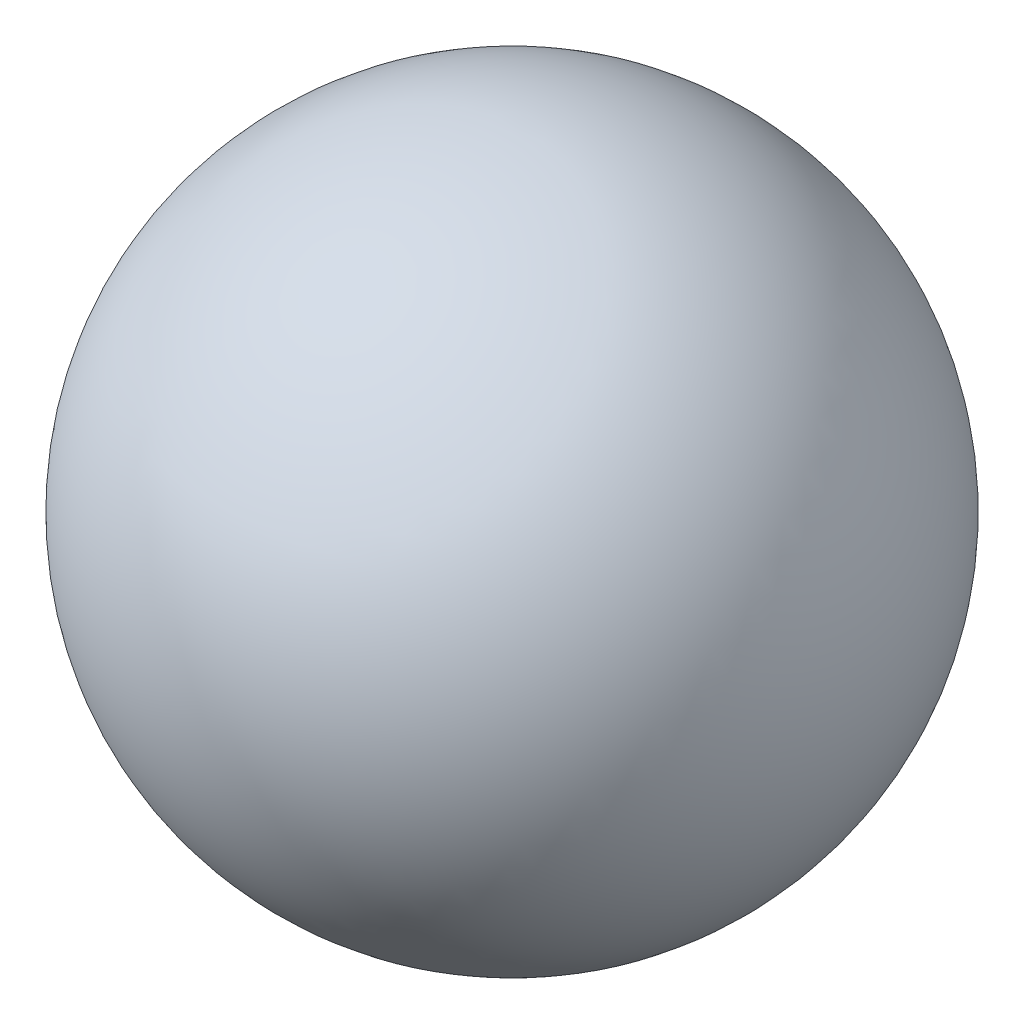
SolidWorks part; units mm, degrees
ref_plane "前视基准面" through (0, 0, 0) normal (0, 0, 1) x (1, 0, 0)
ref_plane "上视基准面" through (0, 0, 0) normal (0, 1, 0) x (1, 0, 0)
ref_plane "右视基准面" through (0, 0, 0) normal (1, 0, 0) x (0, 0, -1)
sketch "草图1" plane through (0, 0, 0) normal (0, 0, 1) x (1, 0, 0)
  line L0 (0, 8) -> (0, -8) construction
  line L1 (0, -8) -> (0, 8)
  arc A0 (0, 8) -> (0, -8) centre (0, 0) ccw
  point P4 (0, 0)
  dimension "D1" = 16
revolve "旋转1" add sketch "草图1" angle 360 about L0
